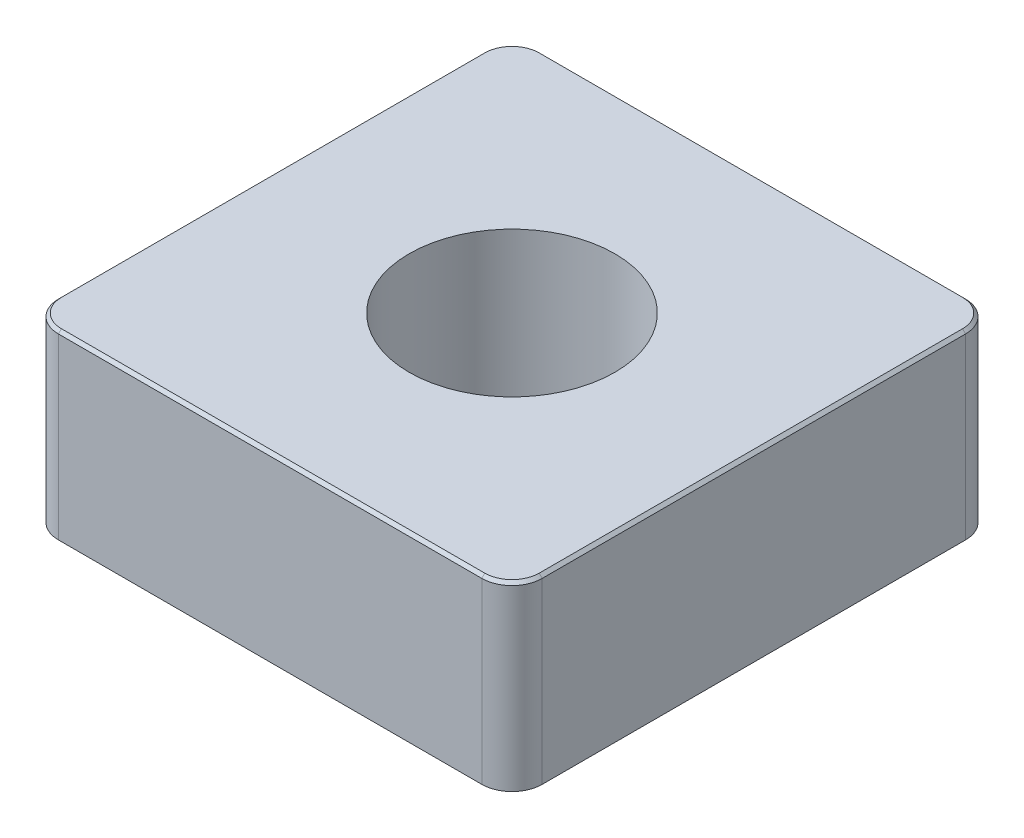
from build123d import *

# Parameters (mm, degrees)
SKETCH1_W              = 80
SKETCH1_H              = 80
BOSS_EXTRUDE1_DEPTH    = 30
M36X2_0_TAPPED_HOLE1_D = 34
FILLET1_R              = 5
CHAMFER1_SIZE          = 0.5


with BuildPart() as part:
    # Sketch1 → Boss-Extrude1 (new body)
    with BuildSketch(Plane(origin=(0, 30, 0), x_dir=(1, 0, 0), z_dir=(0, 1, 0))):
        Rectangle(SKETCH1_W, SKETCH1_H)
    extrude(amount=-BOSS_EXTRUDE1_DEPTH)

    # M36x2.0 Tapped Hole1 (through all)
    with Locations(Plane(origin=(0, 30, 0), x_dir=(1, 0, 0), z_dir=(0, 1, 0))):
        with Locations((0, 0)):
            Hole(M36X2_0_TAPPED_HOLE1_D / 2)

    # Fillet1
    fillet1_edges = [part.edges().sort_by_distance(p)[0] for p in [
        (-40, 15, -40),
        (40, 15, -40),
        (40, 15, 40),
        (-40, 15, 40),
    ]]
    fillet(fillet1_edges, radius=FILLET1_R)

    # Chamfer1
    chamfer1_edges = [part.edges().sort_by_distance(p)[0] for p in [
        (0, 30, 40),
        (-40, 30, 0),
        (40, 30, 0),
        (0, 30, -40),
        (-38.535533906, 30, -38.535533906),
        (38.535533906, 30, -38.535533906),
        (-38.535533906, 30, 38.535533906),
        (38.535533906, 30, 38.535533906),
    ]]
    chamfer(chamfer1_edges, length=CHAMFER1_SIZE)


solid = part.part
